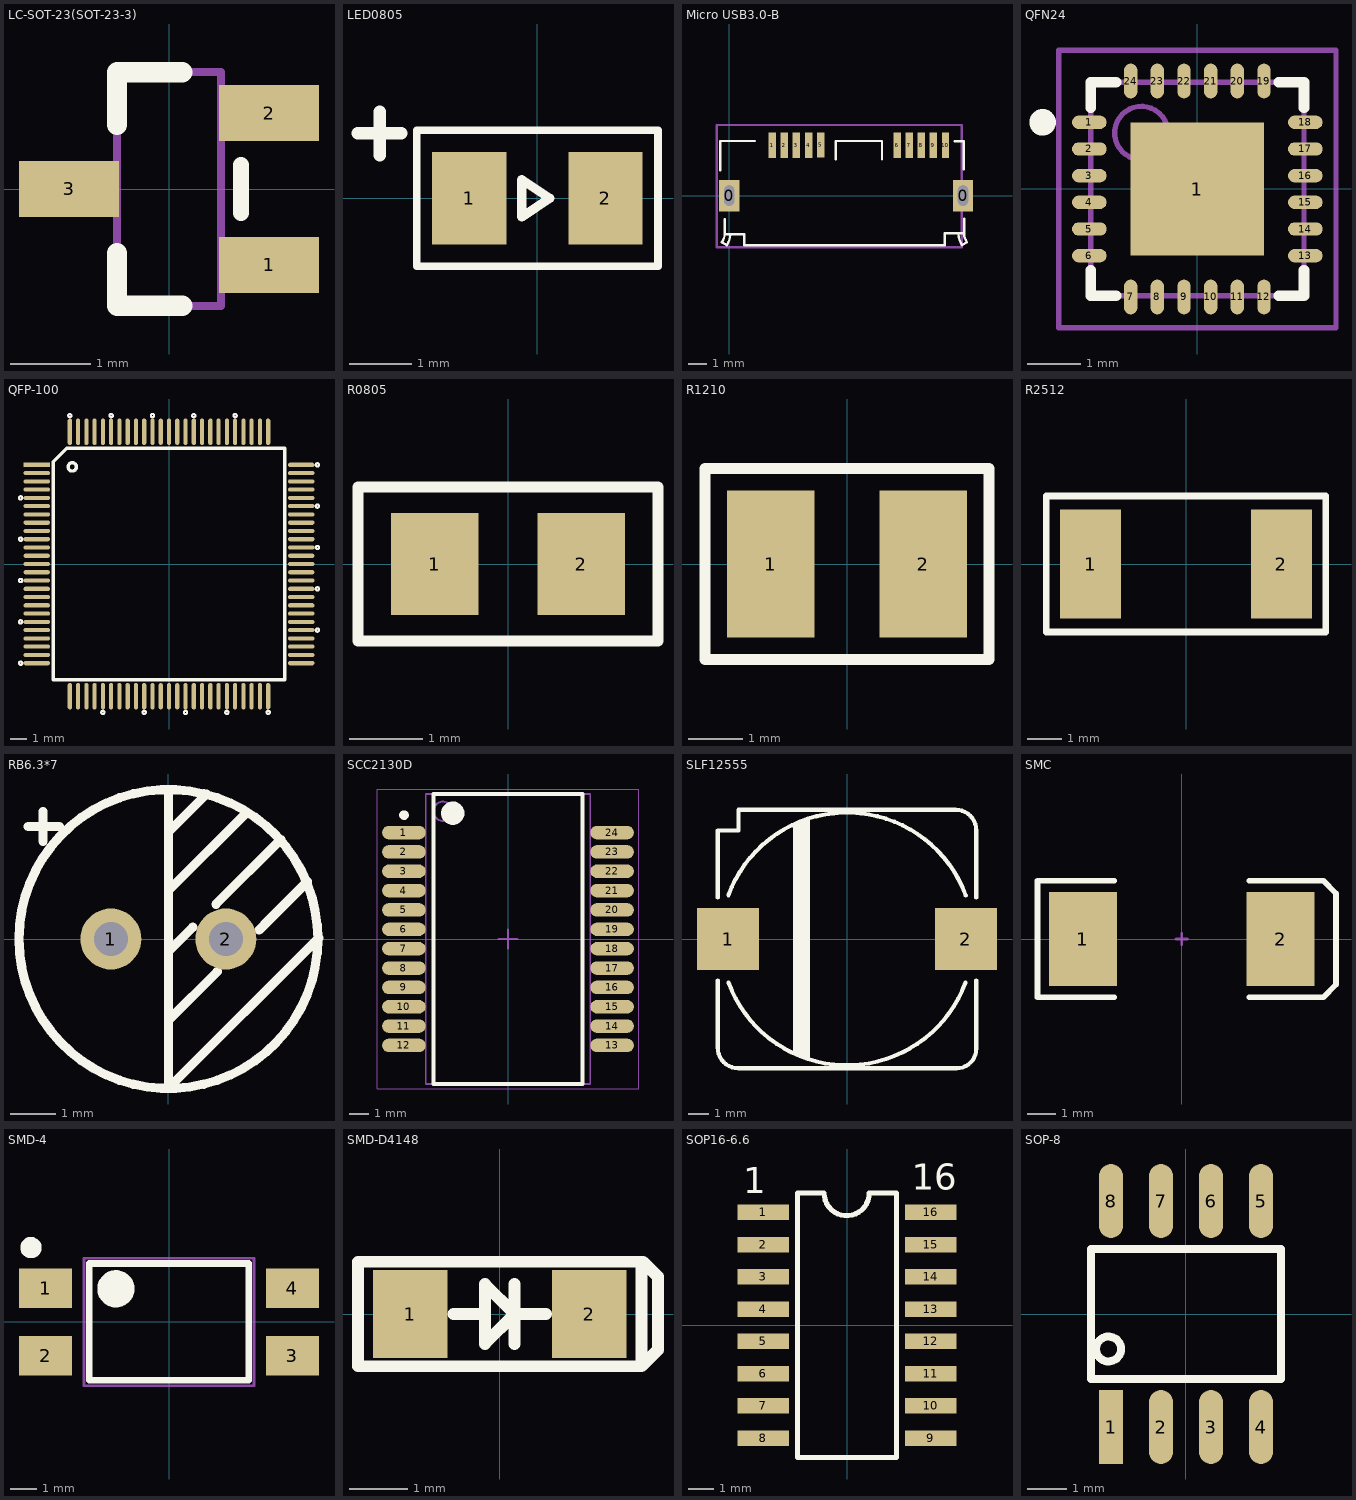
[diagram p0: the footprints below, top view; thin cyan lines are the x and y axes]
# Altium footprint library MISC82155.PcbLib: 38 footprints (part 2 of 3)
Each footprint in its own frame and in the unit in brackets; x right, y up, seen from the top. Pads: shape width x height; smd on the part's side, far side on the other; paste and mask are expansions set on the pad; w line width, h text height; cw(c..) or ccw(c..) is an arc to the next point about the centre after c.

## LC-SOT-23(SOT-23-3) [mm]
pads (3):
  rect 1.25x0.7 smd: 1(1.25,-0.95) 2(1.25,0.95) 3(-1.25,0)
Top Overlay:
  lines w0.2: 0.9,-0.3 0.9,0.3
  lines w0.254: -0.65,-0.8 -0.65,-1.46 0.165,-1.46 ; 0.165,1.46 -0.65,1.46 ; -0.65,0.8 -0.65,1.46 ; -0.65,0.8 -0.65,1.46 ; -0.65,0.8 -0.65,1.46
Mechanical 13:
  lines w0.1: -0.65,-1.46 -0.65,1.46 ; -0.65,-1.46 0.65,-1.46 ; -0.65,-1.46 0.65,-1.46 ; -0.65,-1.46 -0.65,1.46 ; -0.65,-1.46 0.65,-1.46 ; -0.65,-1.46 -0.65,1.46 ; -0.65,1.46 0.65,1.46 ; -0.65,1.46 0.65,1.46 ; -0.65,1.46 0.65,1.46 ; 0.65,-1.46 0.65,1.46 ; 0.65,-1.46 0.65,1.46 ; 0.65,-1.46 0.65,1.46
3D body: height 1.3, standoff 0, extent -1.5,-1.5 1.5,1.5

## LED0805 [mm]
height 3.6
pads (2):
  rect 1.2x1.5 smd: 1(-1.1,0) 2(1.1,0)
Top Overlay:
  lines w0.127: -1.95,-1.1 -1.95,1.1 1.95,1.1 1.95,-1.1 -1.95,-1.1
  lines w0.152: -0.25,-0.3 0.2,0 -0.25,0.3 -0.25,0 -0.25,-0.3
  lines w0.203: -2.9,1.05 -2.55,1.05 ; -2.55,0.7 -2.55,1.05 ; -2.55,1.4 -2.55,1.05 ; -2.2,1.05 -2.55,1.05
3D body: height 0.56, standoff 0, extent -1.016,-0.64 1.016,0.635

## Micro USB3.0-B [mm]
height 1.6
pads (12):
  rect 1.1x1.7 hole 0.55 slot 1.1 at 90 deg: 0(0,0) 0(12.55,0)
  rect 0.4x1.35 smd: 1(2.31,2.7) 2(2.96,2.7) 3(3.61,2.7) 4(4.26,2.703) 5(4.91,2.718) 6(9.01,2.7) 7(9.66,2.7) 8(10.31,2.7) 9(10.96,2.7) 10(11.61,2.7)
Top Overlay:
  lines w0.025: -0.239,-2.055 0.837,-2.055 ; 0.811,-2.055 0.811,-2.332 0.811,-2.655 1.511,-2.655 5.511,-2.655 8.789,-2.655 11.561,-2.655 11.561,-2.505 11.561,-2.182 11.561,-2.055 12.061,-2.055
  lines w0.127: -0.486,1.361 -0.486,2.934 1.368,2.934 ; -0.24,-1.278 -0.24,-2.07 0.801,-2.07 0.801,-2.654 11.571,-2.654 11.571,-2.629 11.571,-2.019 12.612,-2.019 12.612,-1.234 ; -0.239,-2.055 cw(c-0.982,-2.04) -0.317,-2.371 -0.389,-2.505 -0.128,-2.655 -0.044,-2.5 ; -0.037,-2.487 ccw(c-0.806,-2.087) 0.061,-2.095 ; 5.714,1.943 5.714,2.934 8.203,2.934 8.203,1.938 ; 12.111,2.913 12.581,2.913 12.581,1.425 ; 12.311,-2.055 ccw(c13.343,-2.044) 12.428,-2.521 12.5,-2.655 12.761,-2.505 12.689,-2.371 cw(c13.354,-2.04) 12.611,-2.055
Mechanical 1:
  lines w0.127: -0.663,-2.763 12.487,-2.763 12.487,3.787 -0.663,3.787 -0.663,-2.763
3D body: height 2.69, standoff -0.99, extent -0.358,-2.785 12.932,3.115

## QFN24 [mm] "QFN, 24-Leads, Body 4.0x4.0mm (max), Pitch 0.50mm, IPC Medium Density"
height 0.9
pads (25):
  oval 0.65x0.25 smd: 1(-2.025,1.25) 2(-2.025,0.75) 3(-2.025,0.25) 4(-2.025,-0.25) 5(-2.025,-0.75) 6(-2.025,-1.25) 13(2.025,-1.25) 14(2.025,-0.75) 15(2.025,-0.25) 16(2.025,0.25) 17(2.025,0.75) 18(2.025,1.25)
  rect 2.5x2.5 smd: 1(0,0)
  oval 0.25x0.65 smd: 7(-1.25,-2.025) 8(-0.75,-2.025) 9(-0.25,-2.025) 10(0.25,-2.025) 11(0.75,-2.025) 12(1.25,-2.025) 19(1.25,2.025) 20(0.75,2.025) 21(0.25,2.025) 22(-0.25,2.025) 23(-0.75,2.025) 24(-1.25,2.025)
Top Overlay:
  circle w0.25: c-2.9,1.25 r0.125
  lines w0.2: -2,-1.525 -2,-2 -1.525,-2 ; -2,1.525 -2,2 -1.525,2 ; 1.525,-2 2,-2 2,-1.525 ; 1.525,2 2,2 2,1.525
Mechanical 13:
  circle w0.1: c-1.05,1.05 r0.5
  lines w0.1: -2,-2 -2,2 2,2 2,-2 -2,-2
Mechanical 15:
  lines w0.1: -0.5,0 0.5,0 ; 0,-0.5 0,0.5 ; -2.6,-2.6 -2.6,2.6 2.6,2.6 2.6,-2.6 -2.6,-2.6
3D body: height 0.9, standoff 0.02, extent -2,-2 2,2

## QFP-100 [mm]
height 9.5
pads (100):
  rect 1.6x0.254 smd: 1(-8,6)
  oval 1.6x0.254 smd: 2(-8,5.5) 3(-8,5) 4(-8,4.5) 5(-8,4) 6(-8,3.5) 7(-8,3) 8(-8,2.5) 9(-8,2) 10(-8,1.5) 11(-8,1) 12(-8,0.5) 13(-8,0) 14(-8,-0.5) 15(-8,-1) 16(-8,-1.5) 17(-8,-2) 18(-8,-2.5) 19(-8,-3) 20(-8,-3.5) 21(-8,-4) 22(-8,-4.5) 23(-8,-5) 24(-8,-5.5) 25(-8,-6) 51(8,-6) 52(8,-5.5) 53(8,-5) 54(8,-4.5) 55(8,-4) 56(8,-3.5) 57(8,-3) 58(8,-2.5) 59(8,-2) 60(8,-1.5) 61(8,-1) 62(8,-0.5) 63(8,0) 64(8,0.5) 65(8,1) 66(8,1.5) 67(8,2) 68(8,2.5) 69(8,3) 70(8,3.5) 71(8,4) 72(8,4.5) 73(8,5) 74(8,5.5) 75(8,6)
  oval 0.254x1.6 smd: 26(-6,-8) 27(-5.5,-8) 28(-5,-8) 29(-4.5,-8) 30(-4,-8) 31(-3.5,-8) 32(-3,-8) 33(-2.5,-8) 34(-2,-8) 35(-1.5,-8) 36(-1,-8) 37(-0.5,-8) 38(0,-8) 39(0.5,-8) 40(1,-8) 41(1.5,-8) 42(2,-8) 43(2.5,-8) 44(3,-8) 45(3.5,-8) 46(4,-8) 47(4.5,-8) 48(5,-8) 49(5.5,-8) 50(6,-8) 76(6,8) 77(5.5,8) 78(5,8) 79(4.5,8) 80(4,8) 81(3.5,8) 82(3,8) 83(2.5,8) 84(2,8) 85(1.5,8) 86(1,8) 87(0.5,8) 88(0,8) 89(-0.5,8) 90(-1,8) 91(-1.5,8) 92(-2,8) 93(-2.5,8) 94(-3,8) 95(-3.5,8) 96(-4,8) 97(-4.5,8) 98(-5,8) 99(-5.5,8) 100(-6,8)
Top Overlay:
  circle w0.203: c-5.852,5.875 r0.252
  circle w0.127: c-8.975,1.5 r0.1
  circle w0.127: c-8.975,-3.5 r0.1
  circle w0.127: c-8.975,4 r0.1
  circle w0.127: c-8.975,-1 r0.1
  circle w0.127: c-8.975,-6 r0.1
  circle w0.127: c6,-8.975 r0.1
  circle w0.127: c1,-8.975 r0.1
  circle w0.127: c-4,-8.975 r0.1
  circle w0.127: c3.5,-8.975 r0.1
  circle w0.127: c-1.5,-8.975 r0.1
  circle w0.127: c8.975,-1.5 r0.1
  circle w0.127: c8.975,3.5 r0.1
  circle w0.127: c8.975,-4 r0.1
  circle w0.127: c8.975,1 r0.1
  circle w0.127: c8.975,6 r0.1
  circle w0.127: c1.5,8.975 r0.1
  circle w0.127: c-3.5,8.975 r0.1
  circle w0.127: c4,8.975 r0.1
  circle w0.127: c-1,8.975 r0.1
  circle w0.127: c-6,8.975 r0.1
  lines w0.203: -7,-7 -7,6.2 -6.2,7 7,7 7,-7 -7,-7

## R0805 [mm]
pads (2):
  rect 1.2x1.4 smd: 1(-1,0) 2(1,0)
Top Overlay:
  lines w0.152: -2.05,-1.05 2.05,-1.05 2.05,1.05 -2.05,1.05 -2.05,-1.05
3D body: height 0.61, standoff 0, extent -1.016,-0.653 1.016,0.622

## R1210 [mm]
height 3.98
pads (2):
  rect 1.6x2.7 smd: 1(-1.4,0) 2(1.4,0)
Top Overlay:
  lines w0.203: -2.6,-1.75 2.6,-1.75 2.6,1.75 -2.6,1.75 -2.6,-1.75

## R2512 [mm]
height 3.98
pads (2):
  rect 1.8x3.2 smd: 1(-2.8,0) 2(2.8,0)
Top Overlay:
  lines w0.203: -4.1,-2 -4.1,2 4.1,2 4.1,-2 -4.1,-2
3D body: height 0.61, standoff 0, extent -3.175,-1.525 3.175,1.526

## RB6.3*7 [mm]
height 3.98
pads (2):
  round 1.35 hole 0.75: 1(-1.27,0) 2(1.27,0)
Top Overlay:
  circle w0.203: c0,0 r3.302
  lines w0.203: -3.099,2.489 -2.413,2.489 ; -2.769,2.159 -2.769,2.819 ; 0,-1.8 1.079,-0.721 ; 0,-0.3 0,-0.28 0.539,0.259 ; 0,1.067 1.727,2.794 ; 0,2.362 0.838,3.2 ; 0,3.302 0,-3.302 3.327,0.025 ; 1.049,0.769 2.48,2.2 ; 2.003,0.2 3.073,1.27 2.134,0.33 2.13,0.33

## SCC2130D [mm] "SOP, 24-Leads, Body 15.00x8.50mm, Pitch 1.00mm, IPC Medium Density"
height 4.2
pads (24):
  oval 2.25x0.7 smd: 1(-5.375,5.5) 2(-5.375,4.5) 3(-5.375,3.5) 4(-5.375,2.5) 5(-5.375,1.5) 6(-5.375,0.5) 7(-5.375,-0.5) 8(-5.375,-1.5) 9(-5.375,-2.5) 10(-5.375,-3.5) 11(-5.375,-4.5) 12(-5.375,-5.5) 13(5.375,-5.5) 14(5.375,-4.5) 15(5.375,-3.5) 16(5.375,-2.5) 17(5.375,-1.5) 18(5.375,-0.5) 19(5.375,0.5) 20(5.375,1.5) 21(5.375,2.5) 22(5.375,3.5) 23(5.375,4.5) 24(5.375,5.5)
Top Overlay:
  circle w0.25: c-5.375,6.4 r0.125
  circle w0.6: c-2.85,6.5 r0.3
  lines w0.2: -3.85,-7.5 -3.85,7.5 3.85,7.5 3.85,-7.5 -3.85,-7.5
Mechanical 13:
  circle w0.1: c-3.35,6.6 r0.5
  lines w0.1: -4.25,-7.5 -4.25,7.5 4.25,7.5 4.25,-7.5 -4.25,-7.5
Mechanical 15:
  lines w0.05: -6.75,-7.75 -6.75,7.75 6.75,7.75 6.75,-7.75 -6.75,-7.75
  lines w0.1: -0.5,0 0.5,0 ; 0,-0.5 0,0.5
3D body: height 4.2, standoff 0.25, extent -4.25,-7.5 4.25,7.5

## SLF12555 [mm] "TDK SMD power inductor"
height 4.5
pads (2):
  rect 3x3 smd: 1(-5.75,0) 2(5.75,0)
Top Overlay:
  lines w0.2: -6.25,-2 -6.25,-5.25 ccw(c-5.25,-5.25) -5.25,-6.25 5.3,-6.25 ccw(c5.3,-5.3) 6.25,-5.3 6.25,-2 ; -6.25,2 -6.25,5.25 -5.25,5.25 -5.25,6.25 5.25,6.25 cw(c5.25,5.25) 6.25,5.25 6.25,2 ; -5.734,2.118 cw(c0,0) 5.737,2.109 ; -5.726,-2.11 ccw(c0,0) 5.726,-2.11 ; -2.5,-5.55 -2.5,5.55 ; -2.35,-5.6 -2.35,5.6 ; -2.2,-5.65 -2.2,5.65 ; -2.05,-5.65 -2.05,5.7 ; -1.9,-5.75 -1.9,5.75

## SMC [mm] "DO-214-AB/SMC; 2 C-Bend Leads; Body 7.9 x 5.9 mm, inc. leads (LxW)"
height 2.65
pads (2):
  rect 2.4x3.3 smd: 1(-3.475,0) 2(3.475,0)
Top Overlay:
  lines w0.2: -2.375,-2.05 -5.075,-2.05 -5.075,2.05 -2.375,2.05 ; 2.375,-2.05 4.975,-2.05 5.425,-1.6 5.425,1.6 4.975,2.055 ; 2.375,2.05 4.975,2.05
Mechanical 1:
  lines w0.1: -0.2,0 0.2,0 ; 0,-0.2 0,0.2

## SMD-4 [mm]
pads (4):
  rect 2x1.5 smd: 1(-4.65,1.27) 2(-4.65,-1.27) 3(4.65,-1.27) 4(4.65,1.27)
Top Overlay:
  circle w0.7: c-2,1.25 r0.35
  circle w0.4: c-5.2,2.8 r0.2
  lines w0.254: -3,-2.2 3,-2.2 3,2.2 -3,2.2 -3,-2.2
Mechanical 13:
  lines w0.1: -3.2,-2.4 -3.2,2.4 3.2,2.4 3.2,-2.4 -3.2,-2.4
3D body: height 3.9, standoff 0, extent -5.015,-2.416 5.015,2.416

## SMD-D4148 [mm]
height 9.5
pads (2):
  rect 1.27x1.5 smd: 1(-1.524,0) 2(1.524,0)
Top Overlay:
  lines w0.203: -0.787,0 -0.254,0 ; 0.254,-0.508 0.254,0.508 ; 0.787,0 0.254,0 ; 0.254,0 -0.254,-0.508 -0.254,0.508 0.254,0 ; 2.413,-0.889 2.692,-0.61 2.692,0.635 2.438,0.889 2.413,0.889 ; 2.413,-0.889 2.413,0.889 ; 2.413,-0.889 -2.413,-0.889 -2.413,0.889 2.413,0.889

## SOP16-6.6 [mil]
height 374.02
pads (16):
  rect 80x24 smd: 1(-130,175) 2(-130,125) 3(-130,75) 4(-130,25) 5(-130,-25) 6(-130,-75) 7(-130,-125) 8(-130,-175) 9(130,-175) 10(130,-125) 11(130,-75) 12(130,-25) 13(130,25) 14(130,75) 15(130,125) 16(130,175)
Top Overlay:
  lines w8: -76.5,-205 76.5,-205 76.5,205 34.59,205 cw(c-0.5,205) -35.59,205 -76.5,205 -76.5,-205
  text "16" at 100,210 h40
  text "1" at -161,205 h40

## SOP-8 [mil]
height 374.02
pads (8):
  rect 24x74 smd: 1(-75,-113)
  oval 24x74 smd: 2(-25,-113) 3(25,-113) 4(75,-113) 5(75,113) 6(25,113) 7(-25,113) 8(-75,113)
Top Overlay:
  circle w8: c-77.5,-35 r12.5
  lines w8: -95,-65 -95,65 95,65 95,-65 -95,-65